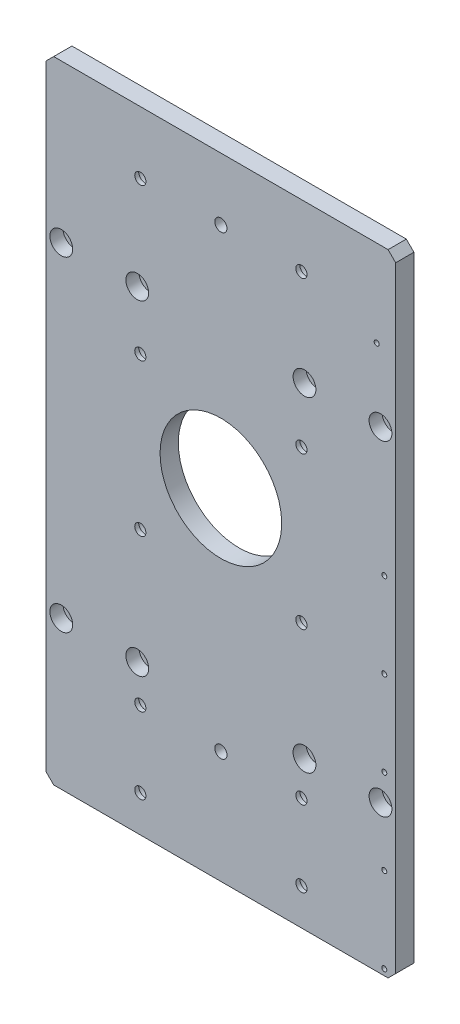
from build123d import *

# Parameters (mm, degrees)
SKETCH_1_W                   = 230
SKETCH_1_H                   = 415
EXTRUDE_1_DEPTH              = 12
CHAMFER_1_SIZE               = 5
HOLE_WIZARD_M8_1_D           = 9
HOLE_WIZARD_M8_1_DEPTH       = 11.5
HOLE_WIZARD_M8_1_CBORE_D     = 15
HOLE_WIZARD_M8_1_CBORE_DEPTH = 8.6
HOLE_WIZARD_M8_1_TIP         = 2.703872786
HOLE_WIZARD_M8_2_D           = 9
HOLE_WIZARD_M8_2_DEPTH       = 22.25
HOLE_WIZARD_M8_2_CBORE_D     = 15
HOLE_WIZARD_M8_2_CBORE_DEPTH = 8.6
HOLE_WIZARD_M8_2_TIP         = 2.703872786
MM_1_D                       = 8
MM_1_DEPTH                   = 22.25
MM_1_TIP                     = 2.403442476
HOLE_WIZARD_M4_1_D           = 3.3
HOLE_WIZARD_M4_2_D           = 3.3
SKETCH_12_R                  = 40
CUT_EXTRUDE_1_DEPTH          = 665.059688056


with BuildPart() as part:
    # 草图1 → 凸台-拉伸1 (new body)
    with BuildSketch(Plane.XY):
        with Locations((95.026115454, 422.357364907)):
            Rectangle(SKETCH_1_W, SKETCH_1_H)
    extrude(amount=EXTRUDE_1_DEPTH)

    # 倒角1
    chamfer_1_edges = [part.edges().sort_by_distance(p)[0] for p in [
        (210.026115454, 214.857364907, 6),
        (-19.973884546, 214.857364907, 6),
        (-19.973884546, 629.857364907, 6),
        (210.026115454, 629.857364907, 6),
    ]]
    chamfer(chamfer_1_edges, length=CHAMFER_1_SIZE)

    # M8 六角凹头螺钉的柱形沉头孔1
    with Locations(Plane(origin=(0, 0, 0), x_dir=(-1, 0, 0), z_dir=(0, 0, -1))):
        with Locations((-148.026115454, 588.857364907), (-42.026115454, 588.857364907), (-148.026115454, 488.857364907), (-42.026115454, 488.857364907), (-148.026115454, 388.857364907), (-42.026115454, 388.857364907), (-148.026115454, 288.857364907), (-42.026115454, 288.857364907), (-148.026115454, 238.857364907), (-42.026115454, 238.857364907)):
            CounterBoreHole(HOLE_WIZARD_M8_1_D / 2, HOLE_WIZARD_M8_1_CBORE_D / 2, HOLE_WIZARD_M8_1_CBORE_DEPTH, depth=HOLE_WIZARD_M8_1_DEPTH)
            with Locations((0, 0, -(HOLE_WIZARD_M8_1_DEPTH + HOLE_WIZARD_M8_1_TIP / 2))):  # 118° drill point
                Cone(0, HOLE_WIZARD_M8_1_D / 2, HOLE_WIZARD_M8_1_TIP, mode=Mode.SUBTRACT)

    # M8 六角凹头螺钉的柱形沉头孔2
    with Locations(Plane.XY.offset(12)):
        with Locations((-9.973884546, 526.357364907), (40.026115454, 526.357364907), (150.026115454, 526.357364907), (200.026115454, 526.357364907), (200.026115454, 312.357364907), (150.026115454, 312.357364907), (40.026115454, 312.357364907), (-9.973884546, 312.357364907)):
            CounterBoreHole(HOLE_WIZARD_M8_2_D / 2, HOLE_WIZARD_M8_2_CBORE_D / 2, HOLE_WIZARD_M8_2_CBORE_DEPTH, depth=HOLE_WIZARD_M8_2_DEPTH)
            with Locations((0, 0, -(HOLE_WIZARD_M8_2_DEPTH + HOLE_WIZARD_M8_2_TIP / 2))):  # 118° drill point
                Cone(0, HOLE_WIZARD_M8_2_D / 2, HOLE_WIZARD_M8_2_TIP, mode=Mode.SUBTRACT)

    # 大小mm 暗销孔1
    with Locations(Plane.XY.offset(12)):
        with Locations((95.026115454, 588.857364907), (95.026115454, 288.857364907)):
            Hole(MM_1_D / 2, depth=MM_1_DEPTH)
            with Locations((0, 0, -(MM_1_DEPTH + MM_1_TIP / 2))):  # 118° drill point
                Cone(0, MM_1_D / 2, MM_1_TIP, mode=Mode.SUBTRACT)

    # M4 螺纹孔1 (through all)
    with Locations(Plane.XY.offset(12)):
        with Locations((202.526115454, 218.857364907), (202.526115454, 274.857364907), (202.526115454, 330.857364907), (202.526115454, 386.857364907), (202.526115454, 442.857364907)):
            Hole(HOLE_WIZARD_M4_1_D / 2)

    # M4 螺纹孔2 (through all)
    with Locations(Plane.XY.offset(12)):
        with Locations((197.526115454, 572.857364907)):
            Hole(HOLE_WIZARD_M4_2_D / 2)

    # 草图12 → 切除-拉伸1 (cut, through all)
    with BuildSketch(Plane(origin=(0, 0, 0), x_dir=(-1, 0, 0), z_dir=(0, 0, -1))):
        with Locations((-95.026115454, 438.857364907)):
            Circle(SKETCH_12_R)
    extrude(amount=-CUT_EXTRUDE_1_DEPTH, mode=Mode.SUBTRACT)


solid = part.part
